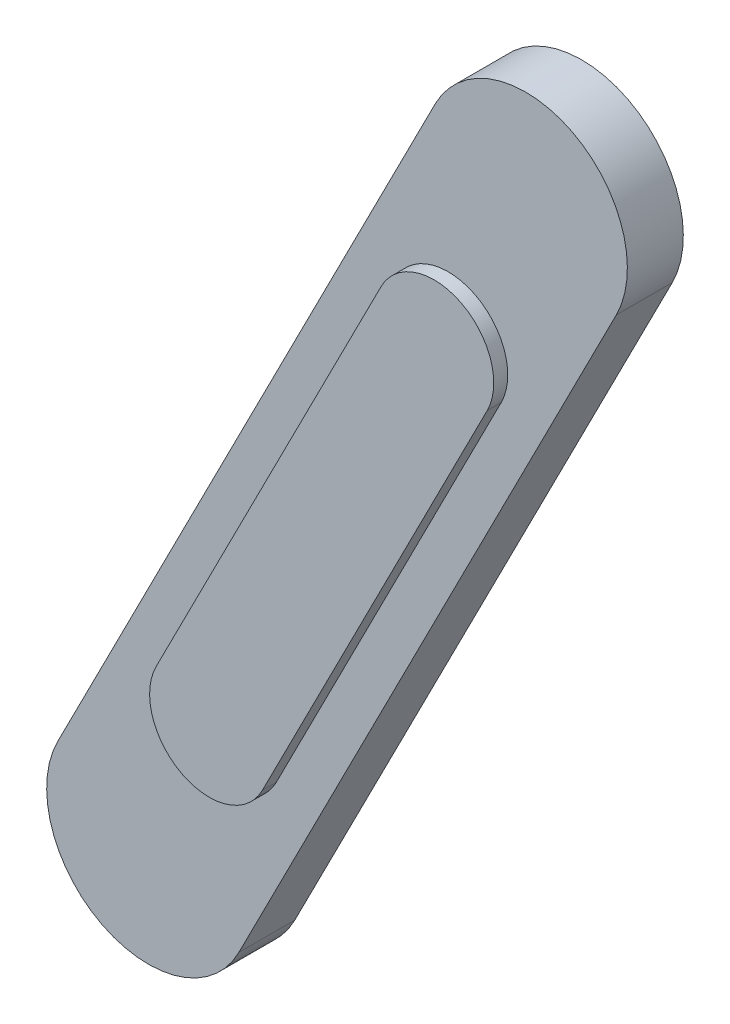
from build123d import *

# Parameters (mm, degrees)
SKETCH2_R           = 1.5
BOSS_EXTRUDE1_DEPTH = 1
BOSS_EXTRUDE2_DEPTH = 0.5
BOSS_EXTRUDE3_START = -0.1
SKETCH4_R           = 1.5
BOSS_EXTRUDE3_DEPTH = 0.1
BOSS_EXTRUDE5_START = -0.1
SKETCH5_R           = 1.5
BOSS_EXTRUDE5_DEPTH = 0.1


with BuildPart() as part:
    # Sketch2 → Boss-Extrude1 (new, symmetric)
    with BuildSketch(Plane.XY):
        with BuildLine():
            Line((-2.378864653, 11.189782176), (11.114395932, 37.671250283))
            ThreePointArc((11.114395932, 37.671250283), (16.00022062, 39.258705834), (17.587676171, 34.372881146))
            Line((17.587676171, 34.372881146), (4.094415586, 7.891413039))
            ThreePointArc((4.094415586, 7.891413039), (-0.791409102, 6.303957488), (-2.378864653, 11.189782176))
        make_face()
        with Locations((0.857775466, 9.540597607)):
            Circle(SKETCH2_R, mode=Mode.SUBTRACT)
        with Locations((14.351036052, 36.022065714)):
            Circle(SKETCH2_R, mode=Mode.SUBTRACT)
    extrude(amount=BOSS_EXTRUDE1_DEPTH, both=True)

    # Sketch3 → Boss-Extrude2 (add, symmetric)
    with BuildSketch(Plane.XY.offset(1)):
        with BuildLine():
            Line((1.637419261, 15.764424462), (9.676771623, 31.542216036))
            ThreePointArc((9.676771623, 31.542216036), (12.542887141, 32.47344695), (13.474118055, 29.607331431))
            Line((13.474118055, 29.607331431), (5.434765693, 13.829539858))
            ThreePointArc((5.434765693, 13.829539858), (2.568650175, 12.898308944), (1.637419261, 15.764424462))
        make_face()
    extrude(amount=BOSS_EXTRUDE2_DEPTH, both=True)

    # Sketch4 → Boss-Extrude3 (add)
    with BuildSketch(Plane.XY.offset(1).offset(BOSS_EXTRUDE3_START)):
        with Locations((0.857775466, 9.540597607)):
            Circle(SKETCH4_R)
    extrude(amount=BOSS_EXTRUDE3_DEPTH)

    # Sketch5 → Boss-Extrude5 (add)
    with BuildSketch(Plane.XY.offset(1).offset(BOSS_EXTRUDE5_START)):
        with Locations((14.351036052, 36.022065714)):
            Circle(SKETCH5_R)
    extrude(amount=BOSS_EXTRUDE5_DEPTH)


solid = part.part
